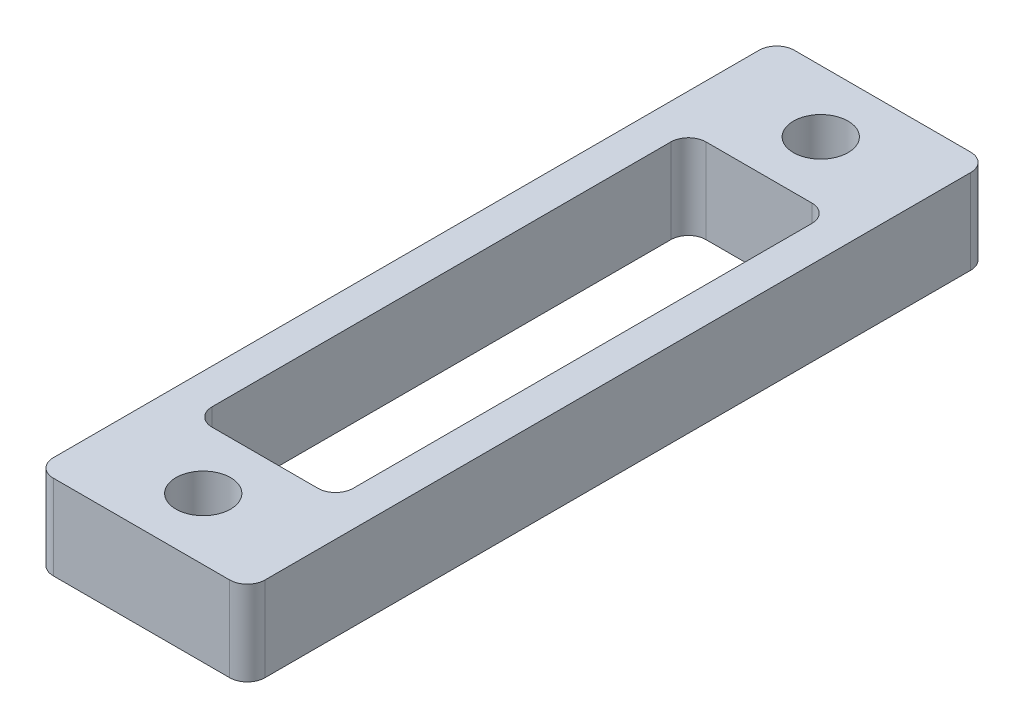
from build123d import *

# Parameters (mm, degrees)
SKETCH_1_W      = 2
SKETCH_1_H      = 28
SKETCH_1_W_2    = 12
SKETCH_1_H_2    = 7
SKETCH_1_R      = 1.55
EXTRUDE_1_DEPTH = 4.8
FILLET_1_R      = 1


with BuildPart() as part:
    # 草图1 → 凸台-拉伸1 (new body)
    # profile 1 of 4: a face of its own
    with BuildSketch(Plane(origin=(0, 0, 0), x_dir=(1, 0, 0), z_dir=(0, 1, 0))):
        with Locations((-5, 17.5)):
            Rectangle(SKETCH_1_W, SKETCH_1_H)
    # profile 2 of 4: a face of its own
    with BuildSketch(Plane(origin=(0, 0, 0), x_dir=(1, 0, 0), z_dir=(0, 1, 0))):
        with Locations((0, 35)):
            Rectangle(SKETCH_1_W_2, SKETCH_1_H_2)
        with Locations(Location((0, 35, 0), (0, 0, 270))):
            Circle(SKETCH_1_R, mode=Mode.SUBTRACT)
    # profile 3 of 4: a face of its own
    with BuildSketch(Plane(origin=(0, 0, 0), x_dir=(1, 0, 0), z_dir=(0, 1, 0))):
        with Locations((5, 17.5)):
            Rectangle(SKETCH_1_W, SKETCH_1_H)
    # profile 4 of 4: a face of its own
    with BuildSketch(Plane(origin=(0, 0, 0), x_dir=(1, 0, 0), z_dir=(0, 1, 0))):
        Rectangle(SKETCH_1_W_2, SKETCH_1_H_2)
        with Locations(Location((0, 0, 0), (0, 0, 270))):
            Circle(SKETCH_1_R, mode=Mode.SUBTRACT)
    extrude(amount=EXTRUDE_1_DEPTH)

    # 圆角1
    fillet_1_edges = [part.edges().sort_by_distance(p)[0] for p in [
        (-4, 2.4, -3.5),
        (4, 2.4, -3.5),
        (4, 2.4, -31.5),
        (-4, 2.4, -31.5),
        (6, 2.4, 3.5),
        (-6, 2.4, 3.5),
        (-6, 2.4, -38.5),
        (6, 2.4, -38.5),
    ]]
    fillet(fillet_1_edges, radius=FILLET_1_R)


solid = part.part
